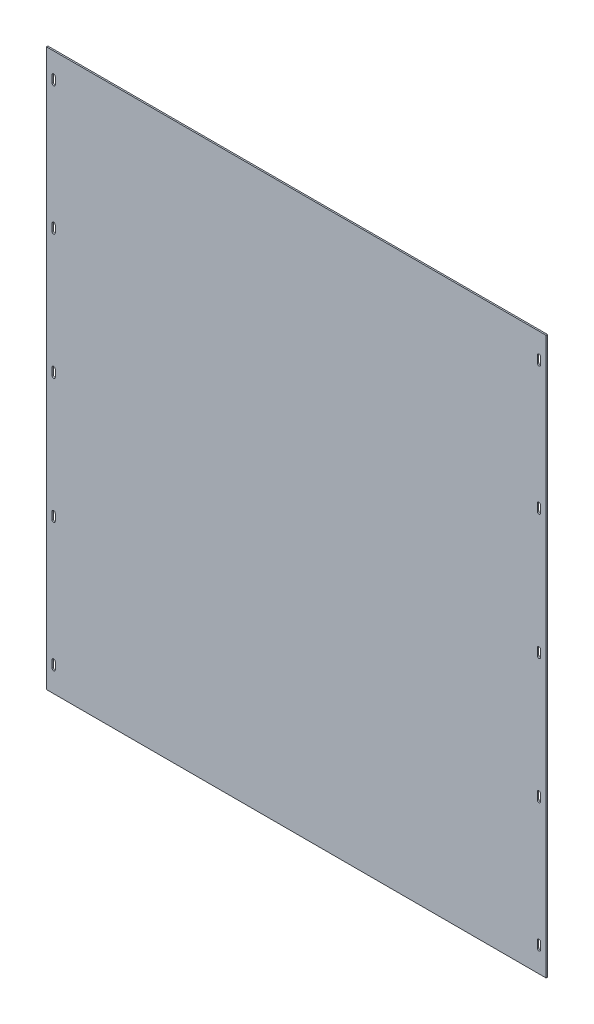
from build123d import *

# Parameters (mm, degrees)
SKETCH_1_W          = 700
SKETCH_1_H          = 780
EXTRUDE_1_DEPTH     = 2
CUT_EXTRUDE_1_DEPTH = 10


with BuildPart() as part:
    # 草图1 → 凸台-拉伸1 (new body)
    with BuildSketch(Plane.XY):
        Rectangle(SKETCH_1_W, SKETCH_1_H)
    extrude(amount=EXTRUDE_1_DEPTH)

    # 草图2 → 切除-拉伸1 (cut)
    with BuildSketch(Plane.XY.offset(2)):
        with BuildLine():
            Line((-337.75, 360), (-337.75, 350))
            ThreePointArc((-337.75, 350), (-340, 347.75), (-342.25, 350))
            Line((-342.25, 350), (-342.25, 360))
            ThreePointArc((-342.25, 360), (-340, 362.25), (-337.75, 360))
        make_face()
        with BuildLine():
            Line((337.75, 360), (337.75, 350))
            ThreePointArc((337.75, 350), (340, 347.75), (342.25, 350))
            Line((342.25, 350), (342.25, 360))
            ThreePointArc((342.25, 360), (340, 362.25), (337.75, 360))
        make_face()
        with BuildLine():
            Line((-342.25, 170), (-342.25, 180))
            ThreePointArc((-342.25, 180), (-340, 182.25), (-337.75, 180))
            Line((-337.75, 180), (-337.75, 170))
            ThreePointArc((-337.75, 170), (-340, 167.75), (-342.25, 170))
        make_face()
        with BuildLine():
            Line((-342.25, -5), (-342.25, 5))
            ThreePointArc((-342.25, 5), (-340, 7.25), (-337.75, 5))
            Line((-337.75, 5), (-337.75, -5))
            ThreePointArc((-337.75, -5), (-340, -7.25), (-342.25, -5))
        make_face()
        with BuildLine():
            Line((342.25, 170), (342.25, 180))
            ThreePointArc((342.25, 180), (340, 182.25), (337.75, 180))
            Line((337.75, 180), (337.75, 170))
            ThreePointArc((337.75, 170), (340, 167.75), (342.25, 170))
        make_face()
        with BuildLine():
            Line((342.25, -5), (342.25, 5))
            ThreePointArc((342.25, 5), (340, 7.25), (337.75, 5))
            Line((337.75, 5), (337.75, -5))
            ThreePointArc((337.75, -5), (340, -7.25), (342.25, -5))
        make_face()
        with BuildLine():
            Line((-342.25, 540), (-342.25, 530))
            ThreePointArc((-342.25, 530), (-340, 527.75), (-337.75, 530))
            Line((-337.75, 530), (-337.75, 540))
            ThreePointArc((-337.75, 540), (-340, 542.25), (-342.25, 540))
        make_face()
        with BuildLine():
            Line((342.25, 540), (342.25, 530))
            ThreePointArc((342.25, 530), (340, 527.75), (337.75, 530))
            Line((337.75, 530), (337.75, 540))
            ThreePointArc((337.75, 540), (340, 542.25), (342.25, 540))
        make_face()
        with BuildLine():
            Line((342.25, -170), (342.25, -180))
            ThreePointArc((342.25, -180), (340, -182.25), (337.75, -180))
            Line((337.75, -180), (337.75, -170))
            ThreePointArc((337.75, -170), (340, -167.75), (342.25, -170))
        make_face()
        with BuildLine():
            Line((-342.25, -170), (-342.25, -180))
            ThreePointArc((-342.25, -180), (-340, -182.25), (-337.75, -180))
            Line((-337.75, -180), (-337.75, -170))
            ThreePointArc((-337.75, -170), (-340, -167.75), (-342.25, -170))
        make_face()
        with BuildLine():
            Line((337.75, -360), (337.75, -350))
            ThreePointArc((337.75, -350), (340, -347.75), (342.25, -350))
            Line((342.25, -350), (342.25, -360))
            ThreePointArc((342.25, -360), (340, -362.25), (337.75, -360))
        make_face()
        with BuildLine():
            Line((-337.75, -360), (-337.75, -350))
            ThreePointArc((-337.75, -350), (-340, -347.75), (-342.25, -350))
            Line((-342.25, -350), (-342.25, -360))
            ThreePointArc((-342.25, -360), (-340, -362.25), (-337.75, -360))
        make_face()
    extrude(amount=-CUT_EXTRUDE_1_DEPTH, mode=Mode.SUBTRACT)


solid = part.part
